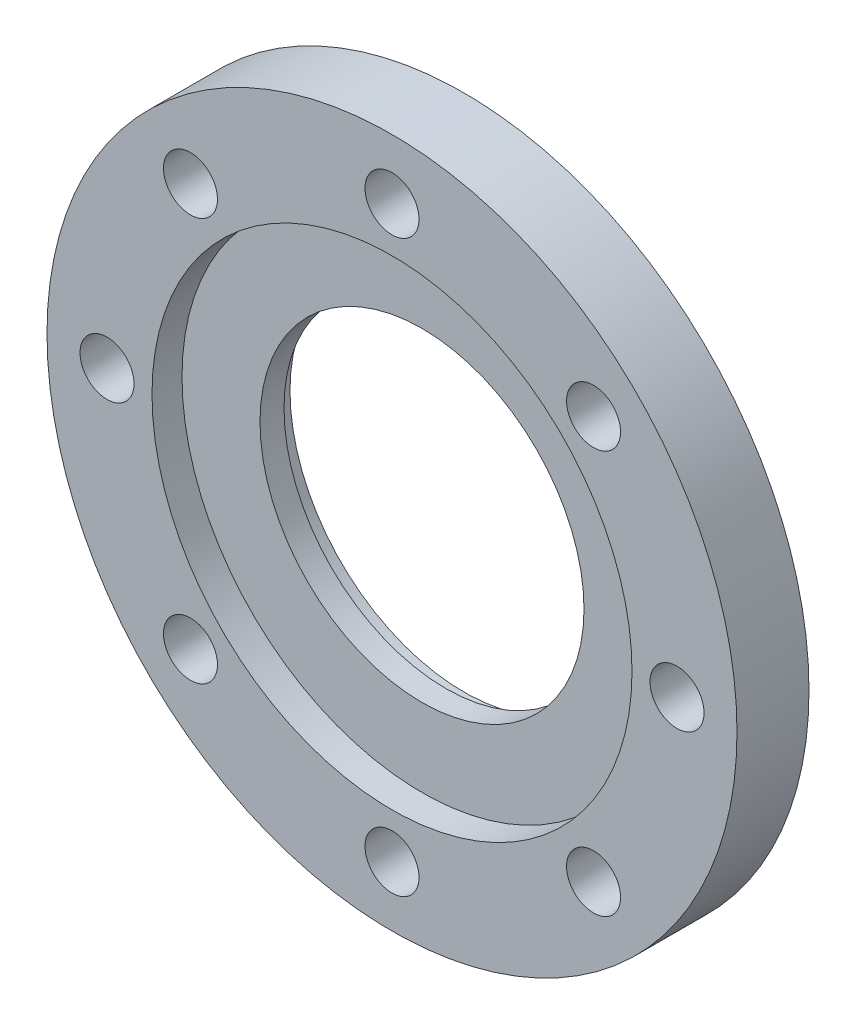
from build123d import *

# Parameters (mm, degrees)
SKETCH_1_R          = 57.5
EXTRUDE_1_DEPTH     = 12
SKETCH_2_R          = 40
CUT_EXTRUDE_1_DEPTH = 5
SKETCH_3_R          = 27
CUT_EXTRUDE_2_DEPTH = 13
SKETCH_4_R          = 29
CUT_EXTRUDE_3_DEPTH = 3
SKETCH_5_R          = 4.5
CUT_EXTRUDE_4_DEPTH = 50


with BuildPart() as part:
    # 草图1 → 凸台-拉伸1 (new body)
    with BuildSketch(Plane.XY):
        Circle(SKETCH_1_R)
    extrude(amount=EXTRUDE_1_DEPTH)

    # 草图2 → 切除-拉伸1 (cut)
    with BuildSketch(Plane.XY.offset(12)):
        Circle(SKETCH_2_R)
    extrude(amount=-CUT_EXTRUDE_1_DEPTH, mode=Mode.SUBTRACT)

    # 草图3 → 切除-拉伸2 (cut)
    with BuildSketch(Plane.XY.offset(7)):
        Circle(SKETCH_3_R)
    extrude(amount=-CUT_EXTRUDE_2_DEPTH, mode=Mode.SUBTRACT)

    # 草图4 → 切除-拉伸3 (cut)
    with BuildSketch(Plane(origin=(0, 0, 0), x_dir=(-1, 0, 0), z_dir=(0, 0, -1))):
        Circle(SKETCH_4_R)
    extrude(amount=-CUT_EXTRUDE_3_DEPTH, mode=Mode.SUBTRACT)

    # 草图5 → 切除-拉伸4 (cut)
    with BuildSketch(Plane.XY.offset(12)):
        with Locations((0, 47.5)):
            Circle(SKETCH_5_R)
        with Locations((33.587572106, 33.587572106)):
            Circle(SKETCH_5_R)
        with Locations((47.5, 0)):
            Circle(SKETCH_5_R)
        with Locations((33.587572106, -33.587572106)):
            Circle(SKETCH_5_R)
        with Locations((0, -47.5)):
            Circle(SKETCH_5_R)
        with Locations((-33.587572106, -33.587572106)):
            Circle(SKETCH_5_R)
        with Locations((-47.5, 0)):
            Circle(SKETCH_5_R)
        with Locations((-33.587572106, 33.587572106)):
            Circle(SKETCH_5_R)
    extrude(amount=-CUT_EXTRUDE_4_DEPTH, mode=Mode.SUBTRACT)


solid = part.part
